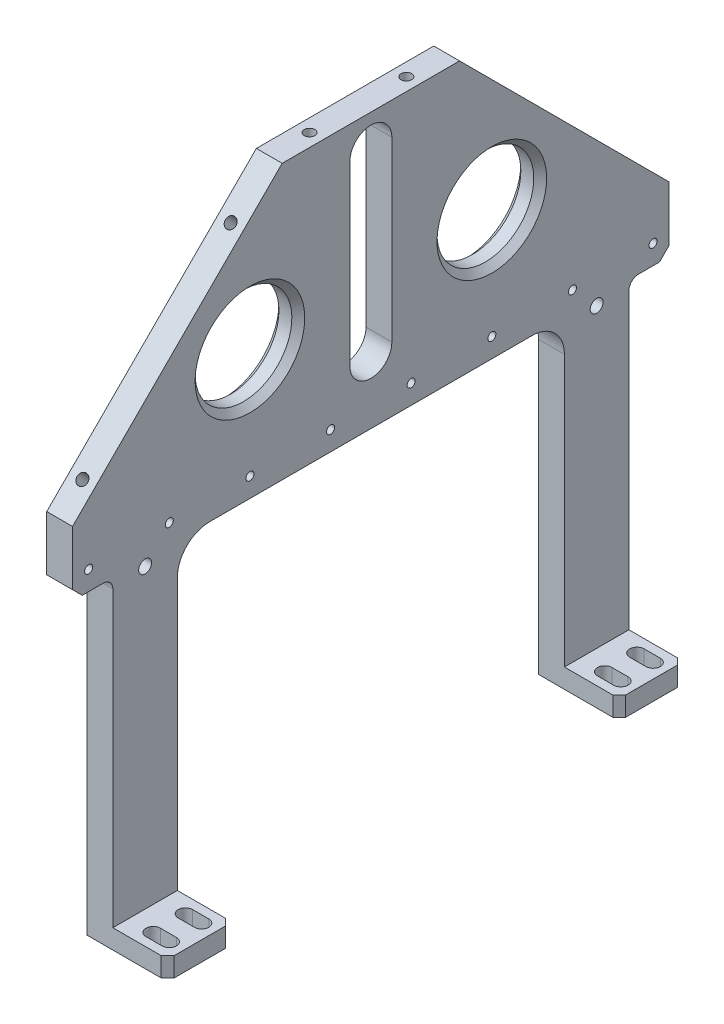
SolidWorks part; units mm, degrees
material "A6061"
ref_plane "Front Plane" through (0, 0, 0) normal (0, 0, 1) x (1, 0, 0)
ref_plane "Top Plane" through (0, 0, 0) normal (0, 1, 0) x (1, 0, 0)
ref_plane "Right Plane" through (0, 0, 0) normal (1, 0, 0) x (0, 0, -1)
sketch "Sketch1" plane through (0, 0, 0) normal (0, 0, 1) x (1, 0, 0)
  line L1 (0, 0) -> (25, 0)
  line L2 (0, 0) -> (0, 185)
  line L3 (0, 185) -> (8, 185)
  line L4 (25, 0) -> (25, 6)
  line L7 (25, 6) -> (8, 6)
  line L8 (8, 185) -> (8, 6)
  dimension "D1" = 6
  dimension "D2" = 185
  dimension "D3" = 8
  dimension "D4" = 25
extrude "Boss-Extrude1" add sketch "Sketch1" along normal mid plane 185
sketch "Sketch16" plane through (0, 0, 0) normal (-1, 0, 0) x (0, 0, 1)
  line L0 (0, 175) -> (0, 120) construction
  line L1 (6.5, 175) -> (6.5, 120)
  line L2 (-6.5, 175) -> (-6.5, 120)
  line L3 (92.5, 185) -> (-92.5, 185) construction
  arc A0 (6.5, 175) -> (-6.5, 175) centre (0, 175) ccw
  arc A1 (-6.5, 120) -> (6.5, 120) centre (0, 120) ccw
  point P3 (0, 147.5)
  dimension "D1" = 6.5
  dimension "D3" = 10
  dimension "D2" = 55
extrude "Cut-Extrude5" cut sketch "Sketch16" against normal through all
hole_wizard "M4 Tapped Hole1" positions "Sketch18" profile "Sketch17" tap size "M4" standard "GB"
sketch "Sketch18" plane through (0, 185, 0) normal (0, 1, 0) x (1, 0, 0)
  line L0 (4, 92.5) -> (4, -45.5766) construction
  line L1 (8, 92.5) -> (0, 92.5) construction
  line L2 (0, 0) -> (23.9353, 0) construction
  point P0 (4, 15)
  point P2 (4, -15)
  dimension "D1" = 30
sketch "Sketch17" plane through (4, 185, -15) normal (1, 0, 0) x (0, 0, 1)
  line L0 (0, 0) -> (0, 11.0914)
  line L1 (0, 11.0914) -> (1.65, 10.1)
  line L2 (1.65, 10.1) -> (1.65, 0)
  line L5 (1.65, 0) -> (0, 0)
  line L10 (0, 11.0914) -> (-1.65, 10.1) construction
  line L11 (0, -6.35) -> (0, 107.95) construction
  dimension "螺纹孔钻头直径" = 3.3
  dimension "螺纹孔钻头深度" = 10.1
  dimension "导头角度" = 118
cosmetic thread "Hole Thread1" parameters "D1"=8, "D2"=4
cosmetic thread "Hole Thread2" parameters "D1"=8, "D2"=4
sketch "Sketch19" plane through (0, 0, 0) normal (-1, 0, 0) x (0, 0, 1)
  line L0 (0, 0) -> (0, 75.0132) construction
  line L1 (92.5, 0) -> (80, 0)
  line L2 (92.5, 0) -> (92.5, 100)
  line L3 (92.5, 100) -> (80, 100)
  line L4 (80, 0) -> (80, 100)
  line L5 (-92.5, 0) -> (-80, 0)
  line L6 (-92.5, 0) -> (-92.5, 100)
  line L7 (-92.5, 100) -> (-80, 100)
  line L8 (-80, 0) -> (-80, 100)
  line L9 (92.5, 185) -> (-92.5, 185) construction
  dimension "D1" = 160
  dimension "D2" = 85
extrude "Cut-Extrude6" cut sketch "Sketch19" against normal through all
sketch "Sketch10" plane through (0, 0, 0) normal (-1, 0, 0) x (0, 0, 1)
  line L0 (80, 0) -> (-80, 0) construction
  line L1 (-60, 0) -> (60, 0)
  line L2 (-60, 0) -> (-60, 100)
  line L3 (-60, 100) -> (60, 100)
  line L4 (60, 0) -> (60, 100)
  line L5 (92.5, 185) -> (-92.5, 185) construction
  line L6 (0, 0) -> (0, 183.8517) construction
  circle A0 centre (37.5, 140) radius 15
  circle A1 centre (-37.5, 140) radius 15
  dimension "D3" = 45
  dimension "D4" = 75
  dimension "D5" = 30
  dimension "D1" = 120
  dimension "D2" = 85
extrude "Cut-Extrude3" cut sketch "Sketch10" against normal through all
hole_wizard "M3 Tapped Hole1" positions "Sketch22" profile "Sketch21" tap size "M3" standard "GB" end condition through all
sketch "Sketch22" plane through (0, 0, 0) normal (-1, 0, 0) x (0, 0, 1)
  line L0 (-92.5, 185) -> (-92.5, 100) construction
  line L1 (-80, 100) -> (-92.5, 100) construction
  point P0 (-87.5, 106)
  point P12 (-62.5, 106)
  point P13 (-37.5, 106)
  point P14 (-12.5, 106)
  point P15 (12.5, 106)
  point P16 (37.5, 106)
  point P17 (62.5, 106)
  point P18 (87.5, 106)
  dimension "D1" = 5
  dimension "D2" = 6
  dimension "D3" = 8
sketch "Sketch21" plane through (0, 106, -87.5) normal (0, 1, 0) x (0, 0, 1)
  line L0 (0, 0) -> (0, 25)
  line L1 (0, 25) -> (1.25, 25)
  line L2 (1.25, 25) -> (1.25, 0)
  line L5 (1.25, 0) -> (0, 0)
  line L11 (0, -6.35) -> (0, 107.95) construction
  dimension "通孔螺纹孔钻头直径" = 2.5
  dimension "通孔螺纹孔钻头深度" = 25
cosmetic thread "Hole Thread3" parameters "D2"=3
cosmetic thread "Hole Thread4" parameters "D2"=3
cosmetic thread "Hole Thread5" parameters "D2"=3
cosmetic thread "Hole Thread6" parameters "D2"=3
cosmetic thread "Hole Thread7" parameters "D2"=3
cosmetic thread "Hole Thread8" parameters "D2"=3
cosmetic thread "Hole Thread9" parameters "D2"=3
cosmetic thread "Hole Thread10" parameters "D2"=3
hole_wizard "Size mm Blind Pin Hole1" positions "Sketch24" profile "Sketch23" hole size "Ø4.0" standard "GB" end condition through all
sketch "Sketch24" plane through (0, 0, 0) normal (-1, 0, 0) x (0, 0, 1)
  line L1 (70, 0) -> (70, 105.9448) construction
  line L2 (80, 0) -> (60, 0) construction
  line L5 (-70, 0) -> (-70, 99.7695) construction
  line L6 (-60, 0) -> (-80, 0) construction
  circle A0 centre (87.5, 106) radius 1.25 construction
  point P0 (-70, 98)
  point P2 (70, 98)
  dimension "D1" = 8
sketch "Sketch23" plane through (0, 98, -70) normal (0, 1, 0) x (0, 0, 1)
  line L0 (0, 0) -> (0, 25)
  line L1 (0, 25) -> (2, 25)
  line L2 (2, 25) -> (2, 0)
  line L5 (2, 0) -> (0, 0)
  line L11 (0, -6.35) -> (0, 107.95) construction
  dimension "通孔孔直径" = 4
  dimension "通孔孔深度" = 25
sketch "Sketch25" plane through (0, 0, 0) normal (0, -1, 0) x (1, 0, 0)
  line L0 (20.5, 75) -> (15.5, 75) construction
  line L1 (20.5, 72.75) -> (15.5, 72.75)
  line L2 (20.5, 77.25) -> (15.5, 77.25)
  line L3 (20.5, 65) -> (15.5, 65) construction
  line L4 (20.5, 62.75) -> (15.5, 62.75)
  line L5 (20.5, 67.25) -> (15.5, 67.25)
  line L6 (20.5, -65) -> (15.5, -65) construction
  line L7 (20.5, -67.25) -> (15.5, -67.25)
  line L8 (20.5, -62.75) -> (15.5, -62.75)
  line L9 (20.5, -75) -> (15.5, -75) construction
  line L10 (20.5, -77.25) -> (15.5, -77.25)
  line L11 (20.5, -72.75) -> (15.5, -72.75)
  line L12 (0, 0) -> (27.7894, 0) construction
  line L13 (25, -70) -> (7.7172, -70) construction
  line L14 (25, -60) -> (25, -80) construction
  line L15 (25, -80) -> (0, -80) construction
  line L16 (25, 70) -> (8.8843, 70) construction
  line L17 (25, 80) -> (25, 60) construction
  arc A0 (20.5, 72.75) -> (20.5, 77.25) centre (20.5, 75) ccw
  arc A1 (15.5, 77.25) -> (15.5, 72.75) centre (15.5, 75) ccw
  arc A2 (20.5, 62.75) -> (20.5, 67.25) centre (20.5, 65) ccw
  arc A3 (15.5, 67.25) -> (15.5, 62.75) centre (15.5, 65) ccw
  arc A4 (20.5, -67.25) -> (20.5, -62.75) centre (20.5, -65) ccw
  arc A5 (15.5, -62.75) -> (15.5, -67.25) centre (15.5, -65) ccw
  arc A6 (20.5, -77.25) -> (20.5, -72.75) centre (20.5, -75) ccw
  arc A7 (15.5, -72.75) -> (15.5, -77.25) centre (15.5, -75) ccw
  point P2 (18, 75)
  point P7 (18, 65)
  point P14 (18, -65)
  point P21 (18, -75)
  dimension "D1" = 5
  dimension "D2" = 4.5
  dimension "D4" = 2.25
  dimension "D3" = 5
extrude "Cut-Extrude7" cut sketch "Sketch25" against normal through all
chamfer "Chamfer2" distance 65 angle 45 2 edges at (4, 185, -92.5) (4, 185, 92.5)
chamfer "Chamfer3" distance 3 angle 45 2 edges at (4, 100, -92.5) (4, 100, 92.5)
chamfer "Chamfer4" distance 2 angle 45 8 edges at (25, 3, -80) (25, 3, -60) (25, 3, 60) (25, 3, 80) (0, 140, 52.5) (8, 125, 37.5) (0, 140, -22.5) (8, 125, -37.5)
fillet "Fillet1" radius 10 2 edges at (4, 100, 60) (4, 100, -60)
fillet "Fillet2" radius 3 2 edges at (4, 100, 80) (4, 100, -80)
hole_wizard "M4 Tapped Hole2" positions "Sketch27" profile "Sketch26" tap size "M4" standard "GB"
sketch "Sketch27" plane through (0, 106.25, -106.25) normal (0, 0.7071, -0.7071) x (-1, 0, 0)
  line L0 (-4, 111.3693) -> (-4, 55.0978) construction
  line L1 (-8, 111.3693) -> (0, 111.3693) construction
  line L2 (0, 19.4454) -> (-8, 19.4454) construction
  point P0 (-4, 94.4454)
  point P2 (-4, 29.4454)
  dimension "D1" = 65
  dimension "D2" = 10
cosmetic thread "Hole Thread11" parameters "D1"=8, "D2"=4
cosmetic thread "Hole Thread12" parameters "D1"=8, "D2"=4
sketch "Sketch26" plane through (4, 173.033, -39.467) normal (1, 0, 0) x (0, 0.7071, 0.7071)
  line L0 (0, 0) -> (0, 11.0914)
  line L1 (0, 11.0914) -> (1.65, 10.1)
  line L2 (1.65, 10.1) -> (1.65, 0)
  line L5 (1.65, 0) -> (0, 0)
  line L10 (0, 11.0914) -> (-1.65, 10.1) construction
  line L11 (0, -6.35) -> (0, 107.95) construction
  dimension "螺纹孔钻头直径" = 3.3
  dimension "螺纹孔钻头深度" = 10.1
  dimension "导头角度" = 118
mirror "Mirror1" about plane through (0, 0, 0) normal (0, 0, 1) of "M4 Tapped Hole2"
